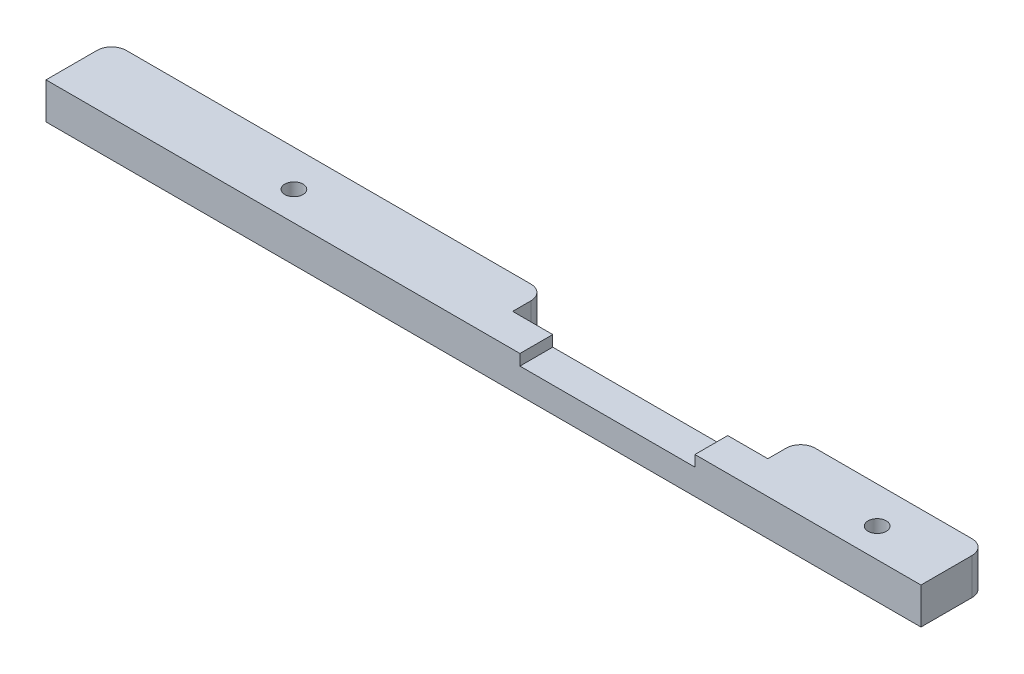
SolidWorks part; units mm, degrees
ref_plane "Front Plane" through (0, 0, 0) normal (0, 0, 1) x (1, 0, 0)
ref_plane "Top Plane" through (0, 0, 0) normal (0, 1, 0) x (1, 0, 0)
ref_plane "Right Plane" through (0, 0, 0) normal (1, 0, 0) x (0, 0, -1)
sketch "Sketch1" plane through (0, 0, 0) normal (0, 1, 0) x (1, 0, 0)
  line L0 (0, 0) -> (0, 9)
  line L1 (0, 9) -> (120, 9)
  line L2 (120, 9) -> (120, 0)
  line L3 (120, 0) -> (0, 0)
  dimension "D1" = 9
  dimension "D2" = 120
extrude "Boss-Extrude1" add sketch "Sketch1" along normal blind 5
hole_wizard "M3 Tapped Hole1" positions "Sketch3" profile "Sketch2" tap size "M3" standard "GB"
sketch "Sketch3" plane through (0, 5, 0) normal (0, 1, 0) x (-1, 0, 0)
  line L0 (0, -9) -> (0, 0) construction
  line L2 (0, 0) -> (-120, 0) construction
  point P0 (-30, -4)
  point P1 (-110, -4)
  dimension "D1" = 80
  dimension "D2" = 30
  dimension "D3" = 4
sketch "Sketch2" plane through (30, 5, -4) normal (1, 0, 0) x (0, 0, 1)
  line L0 (0, 0) -> (0, 8.5)
  line L1 (0, 8.5) -> (1.25, 8.5)
  line L2 (1.25, 8.5) -> (1.25, 0)
  line L5 (1.25, 0) -> (0, 0)
  line L10 (0, 8.5) -> (-1.25, 8.5) construction
  line L11 (0, -6.35) -> (0, 107.95) construction
  dimension "螺纹孔钻头直径" = 2.5
  dimension "螺纹孔钻头深度" = 8.5
  dimension "导头角度" = 180
cosmetic thread "Cosmetic Thread2" parameters "D1"=5, "D2"=3
cosmetic thread "Cosmetic Thread3" parameters "D1"=5, "D2"=3
sketch "Sketch4" plane through (0, 5, 0) normal (0, 1, 0) x (-1, 0, 0)
  line L0 (-120, -9) -> (0, -9) construction
  line L1 (-94.5, -9) -> (-59.5, -9)
  line L2 (-94.5, -9) -> (-94.5, -4.5)
  line L3 (-94.5, -4.5) -> (-59.5, -4.5)
  line L4 (-59.5, -9) -> (-59.5, -4.5)
  line L5 (-120, 0) -> (-120, -9) construction
  dimension "D1" = 4.5
  dimension "D2" = 25.5
  dimension "D3" = 35
fillet "Fillet1" radius 2 2 edges at (0, 2.5, -9) (120, 2.5, -9)
extrude "Cut-Extrude1" cut sketch "Sketch4" against normal through all
fillet "Fillet2" radius 2 2 edges at (94.5, 2.5, -9) (59.5, 2.5, -9)
sketch "Sketch5" plane through (0, 5, 0) normal (0, -1, 0) x (1, 0, 0)
  line L0 (59.5, -4.5) -> (94.5, -4.5) construction
  line L1 (89, -9) -> (65, -9)
  line L2 (89, -9) -> (89, 0)
  line L3 (89, 0) -> (65, 0)
  line L4 (65, -9) -> (65, 0)
  line L5 (89, -9) -> (65, 0) construction
  line L6 (89, 0) -> (65, -9) construction
  line L7 (0, 0) -> (120, 0) construction
  point P0 (77, -4.5)
  dimension "D1" = 24
extrude "Cut-Extrude2" cut sketch "Sketch5" along normal blind 1.5
